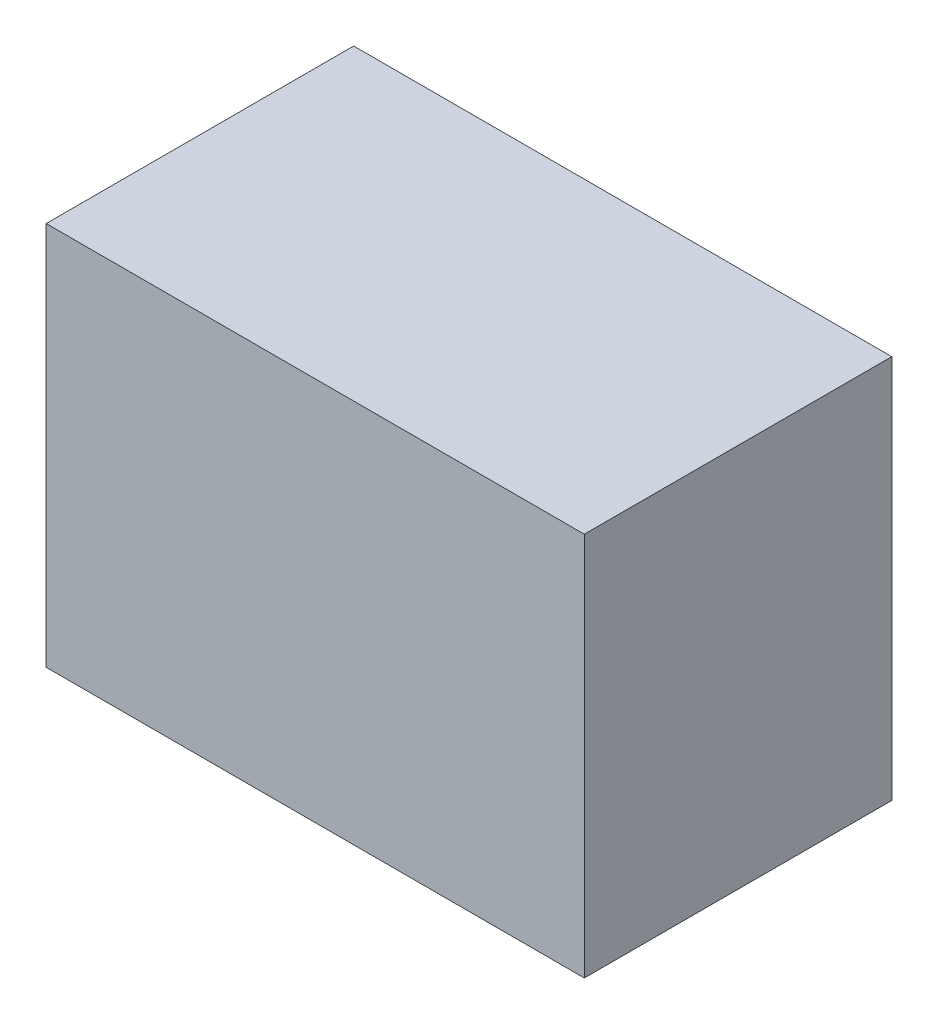
from build123d import *

# Parameters (mm, degrees)
SKETCH_1_W      = 28
SKETCH_1_H      = 20
EXTRUDE_1_DEPTH = 8


with BuildPart() as part:
    # 草图1 → 凸台-拉伸1 (new, symmetric)
    with BuildSketch(Plane.XY):
        Rectangle(SKETCH_1_W, SKETCH_1_H)
    extrude(amount=EXTRUDE_1_DEPTH, both=True)


solid = part.part
